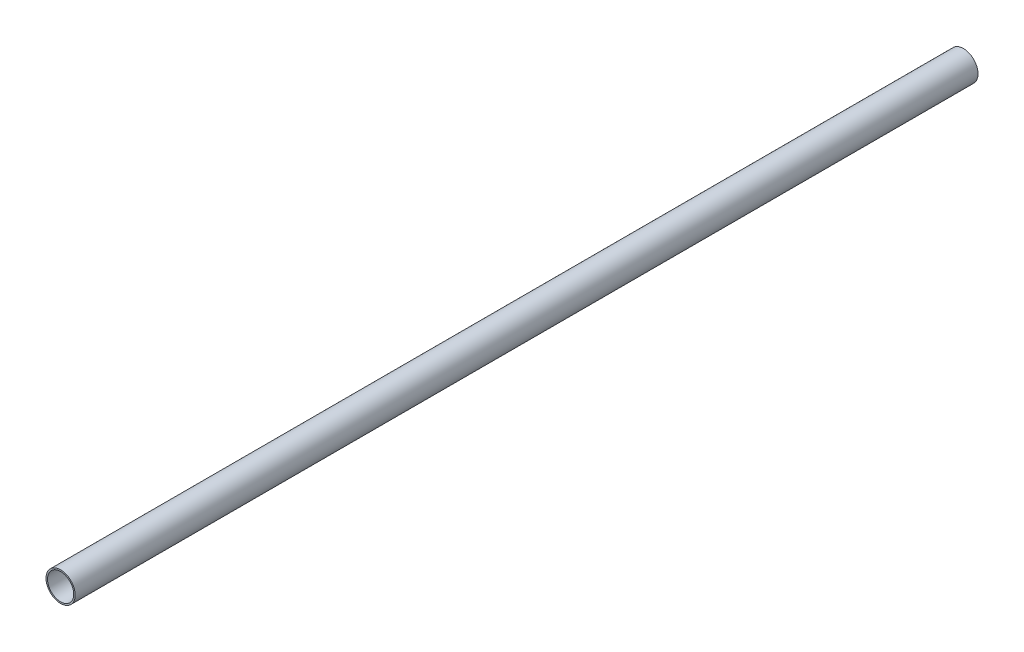
SolidWorks part; units mm, degrees
material "1023 碳钢板 (SS)"
ref_plane "Front Plane" through (0, 0, 0) normal (0, 0, 1) x (1, 0, 0)
ref_plane "Top Plane" through (0, 0, 0) normal (0, 1, 0) x (1, 0, 0)
ref_plane "Right Plane" through (0, 0, 0) normal (1, 0, 0) x (0, 0, -1)
sketch "Sketch1" plane through (0, 0, 0) normal (0, 0, 1) x (1, 0, 0)
  circle A0 centre (0, 0) radius 31.75
  dimension "D1" = 63.5
extrude "Boss-Extrude1" add sketch "Sketch1" along normal blind 1964
shell "Shell1" thickness 3.2
